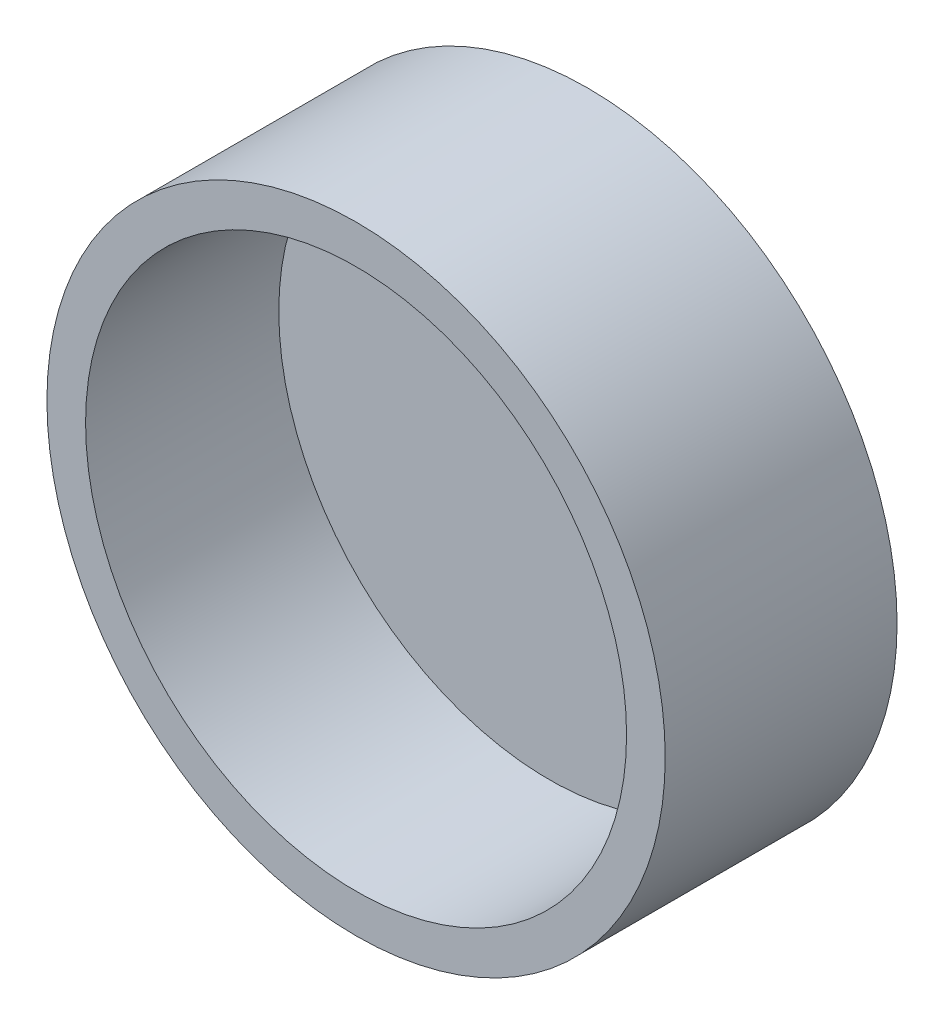
from build123d import *

# Parameters (mm, degrees)
SKETCH1_R           = 40
BOSS_EXTRUDE1_DEPTH = 5
SKETCH2_R           = 40
SKETCH2_R_2         = 35
BOSS_EXTRUDE2_DEPTH = 25


with BuildPart() as part:
    # Sketch1 → Boss-Extrude1 (new body)
    with BuildSketch(Plane.XY):
        Circle(SKETCH1_R)
    extrude(amount=BOSS_EXTRUDE1_DEPTH)

    # Sketch2 → Boss-Extrude2 (add)
    with BuildSketch(Plane.XY.offset(5)):
        Circle(SKETCH2_R)
        Circle(SKETCH2_R_2, mode=Mode.SUBTRACT)
    extrude(amount=BOSS_EXTRUDE2_DEPTH)


solid = part.part
